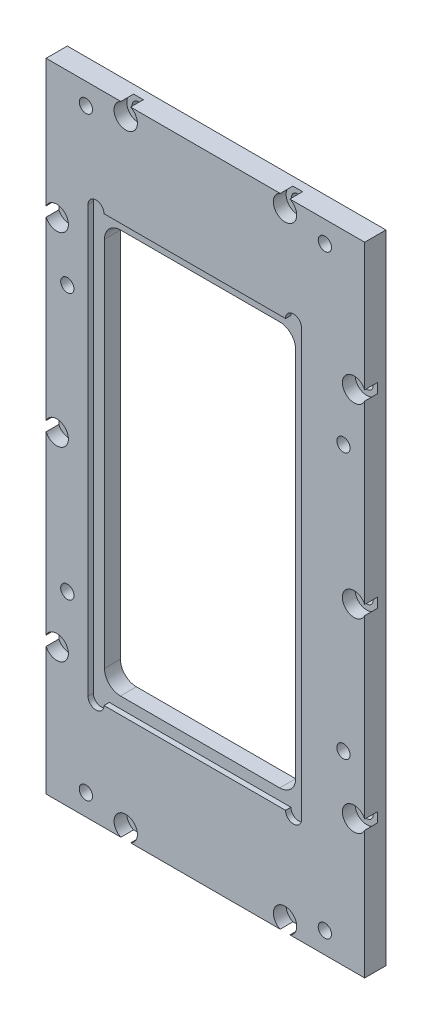
SolidWorks part; units mm, degrees
material "6061Al"
ref_plane "前视基准面" through (0, 0, 0) normal (0, 0, 1) x (1, 0, 0)
ref_plane "上视基准面" through (0, 0, 0) normal (0, 1, 0) x (1, 0, 0)
ref_plane "右视基准面" through (0, 0, 0) normal (1, 0, 0) x (0, 0, -1)
sketch "草图1" plane through (0, 0, 0) normal (0, 0, 1) x (1, 0, 0)
  line L1 (-30, -60) -> (30, -60)
  line L2 (-30, -60) -> (-30, 60)
  line L3 (-30, 60) -> (30, 60)
  line L4 (30, -60) -> (30, 60)
  line L5 (-30, -60) -> (30, 60) construction
  line L6 (-30, 60) -> (30, -60) construction
  point P0 (0, 0)
  dimension "D1" = 120
  dimension "D2" = 60
extrude "凸台-拉伸1" add sketch "草图1" along normal mid plane 4
sketch "草图2" plane through (0, 0, 2) normal (0, 0, 1) x (1, 0, 0)
  line L0 (0, 0) -> (30, 0) construction
  line L1 (30, -60) -> (30, 60) construction
  line L2 (-30, 60) -> (-30, -60) construction
  line L3 (-20, 38) -> (16, 38)
  line L4 (-20, 38) -> (-20, -38)
  line L5 (-20, -38) -> (16, -38)
  line L6 (16, 38) -> (16, -38)
  dimension "D1" = 36
  dimension "D2" = 76
  dimension "D3" = 10
extrude "切除-拉伸1" cut sketch "草图2" against normal through all
sketch "草图3" plane through (0, 0, 2) normal (0, 0, 1) x (1, 0, 0)
  line L8 (18.1, 40.1) -> (-22.1, 40.1)
  line L9 (18.1, -40.1) -> (18.1, 40.1)
  line L10 (-22.1, -40.1) -> (18.1, -40.1)
  line L11 (-22.1, 40.1) -> (-22.1, -40.1)
  line L12 (18.1, 40.1) -> (-22.1, 40.1)
  line L13 (18.1, -40.1) -> (18.1, 40.1)
  line L14 (-22.1, -40.1) -> (18.1, -40.1)
  line L15 (-22.1, 40.1) -> (-22.1, -40.1)
  dimension "D1" = 2.1
extrude "切除-拉伸2" cut sketch "草图3" against normal blind 1
hole_wizard "Ø3.0 (3) 直径孔1" positions "草图4" profile "草图5" hole size "Ø3.0" standard "ISO" end condition up to next
sketch "草图4" plane through (0, 0, 2) normal (0, 0, 1) x (1, 0, 0)
  line L0 (18.1, 40.1) -> (-22.1, 40.1) construction
  line L1 (-22.1, 40.1) -> (-22.1, -40.1) construction
  line L8 (-30, 0) -> (30, 0) construction
  line L9 (-30, 60) -> (-30, -60) construction
  line L10 (30, -60) -> (30, 60) construction
  line L12 (-2, 38) -> (-2, 73.6475) construction
  line L13 (-20, 38) -> (16, 38) construction
  point P0 (-20.6, 40.1)
  point P17 (16.6, 40.1)
  point P39 (16.6, -40.1)
  point P40 (-20.6, -40.1)
  dimension "D1" = 1.5
sketch "草图5" plane through (-20.6, 40.1, 2) normal (1, 0, 0) x (0, -1, 0)
  line L0 (0, 0) -> (0, 1)
  line L1 (0, 1) -> (1.5, 1)
  line L2 (1.5, 1) -> (1.5, 0)
  line L5 (1.5, 0) -> (0, 0)
  line L11 (0, -6.35) -> (0, 107.95) construction
  dimension "通孔孔直径" = 3
  dimension "通孔孔深度" = 1
fillet "圆角1" radius 3 4 edges at (16, 38, -0.5) (16, -38, -0.5) (-20, -38, -0.5) (-20, 38, -0.5)
hole_wizard "M2 六角凹头螺钉的柱形沉头孔1" positions "草图6" profile "草图7" counterbore size "M2" standard "ISO" end condition through all
sketch "草图6" plane through (0, 0, 2) normal (0, 0, 1) x (1, 0, 0)
  point P9 (-28, 0)
  point P21 (-28, 0)
  point P23 (28, 0)
  point P27 (-15, 58)
  point P30 (15, 58)
  point P33 (-28, 35)
  point P36 (28, 35)
  point P39 (-28, -35)
  point P42 (28, -35)
  point P46 (-15, -58)
  point P49 (15, -58)
sketch "草图7" plane through (-28, 0, 2) normal (1, 0, 0) x (0, -1, 0)
  line L0 (0, 0) -> (0, 4)
  line L1 (0, 4) -> (1.2, 4)
  line L3 (1.2, 4) -> (1.2, 2.4)
  line L4 (1.2, 2.4) -> (2.2, 2.4)
  line L5 (2.2, 2.4) -> (2.2, 0)
  line L7 (2.2, 0) -> (0, 0)
  line L11 (0, -6.35) -> (0, 107.95) construction
  dimension "通孔孔直径" = 2.4
  dimension "通孔孔深度" = 4
  dimension "柱形沉头孔直径" = 4.4
  dimension "柱形沉头孔深度" = 2.4
hole_wizard "M3 螺纹孔1" positions "草图9" profile "草图10" tap size "M3" standard "ISO" end condition up to next
sketch "草图9" plane through (0, 0, 2) normal (0, 0, 1) x (1, 0, 0)
  line L0 (0, 60) -> (0, 74.7314) construction
  line L4 (-30, 34.0835) -> (-30, 0.9165) construction
  line L5 (0, 0) -> (48.9555, 0) construction
  line L7 (0, -60) -> (0, -74.7314) construction
  line L8 (14.0835, 60) -> (-14.0835, 60) construction
  line L9 (30, 60) -> (15.9165, 60) construction
  point P2 (-22.5, 56)
  point P4 (22.5, 56)
  point P6 (-26, 25)
  point P8 (26, 25)
  point P27 (26, -25)
  point P28 (-26, -25)
  point P29 (22.5, -56)
  point P30 (-22.5, -56)
  dimension "D1" = 4
  dimension "D2" = 45
  dimension "D3" = 4
  dimension "D4" = 35
sketch "草图10" plane through (-22.5, 56, 2) normal (1, 0, 0) x (0, -1, 0)
  line L0 (0, 0) -> (0, 4)
  line L1 (0, 4) -> (1.25, 4)
  line L2 (1.25, 4) -> (1.25, 0)
  line L5 (1.25, 0) -> (0, 0)
  line L11 (0, -6.35) -> (0, 107.95) construction
  dimension "通孔螺纹孔钻头直径" = 2.5
  dimension "通孔螺纹孔钻头深度" = 4
cosmetic thread "孔螺蚊线1" parameters "D2"=3
cosmetic thread "孔螺蚊线2" parameters "D2"=3
cosmetic thread "孔螺蚊线3" parameters "D2"=3
cosmetic thread "孔螺蚊线4" parameters "D2"=3
cosmetic thread "孔螺蚊线5" parameters "D2"=3
cosmetic thread "孔螺蚊线6" parameters "D2"=3
cosmetic thread "孔螺蚊线7" parameters "D2"=3
cosmetic thread "孔螺蚊线8" parameters "D2"=3
